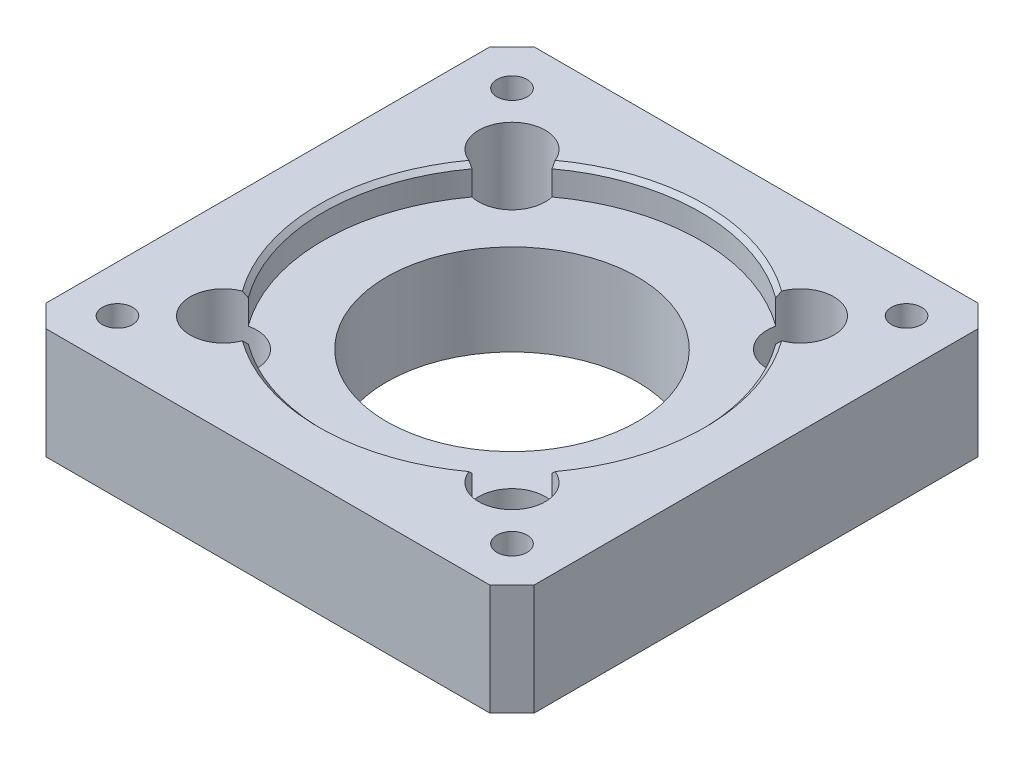
from build123d import *

# Parameters (mm, degrees)
SKETCH_1_W                     = 110
SKETCH_1_H                     = 110
EXTRUDE_1_DEPTH                = 25
SKETCH_3_R                     = 31.25
SKETCH_3_R_2                   = 28.25
EXTRUDE_2_DEPTH                = 2
SKETCH_4_R                     = 28.25
CUT_EXTRUDE_1_DEPTH            = 82.700673192
SKETCH_5_R                     = 42.5
CUT_EXTRUDE_2_DEPTH            = 6.5
HOLE_WIZARD_M8_1_D             = 6.8
HOLE_WIZARD_M8_1_DEPTH         = 19.75
HOLE_WIZARD_M8_1_TIP           = 2.042926105
HOLE_WIZARD_M8_1_2_D           = 9
HOLE_WIZARD_M8_1_2_CBORE_D     = 15
HOLE_WIZARD_M8_1_2_CBORE_DEPTH = 18
CHAMFER_1_SIZE                 = 5
CHAMFER_2_SIZE                 = 1
CHAMFER_3_SIZE                 = 0.5


with BuildPart() as part:
    # 草图1 → 凸台-拉伸1 (new body)
    with BuildSketch(Plane(origin=(0, 0, 0), x_dir=(1, 0, 0), z_dir=(0, 1, 0))):
        Rectangle(SKETCH_1_W, SKETCH_1_H)
    extrude(amount=EXTRUDE_1_DEPTH)

    # 草图3 → 凸台-拉伸2 (add)
    with BuildSketch(Plane.XZ):
        with Locations(Location((0, 0, 0), (0, 0, 270))):
            Circle(SKETCH_3_R)
        with Locations(Location((0, 0, 0), (0, 0, 270))):
            Circle(SKETCH_3_R_2, mode=Mode.SUBTRACT)
    extrude(amount=EXTRUDE_2_DEPTH)

    # 草图4 → 切除-拉伸1 (cut, through all)
    with BuildSketch(Plane.XZ):
        with Locations(Location((0, 0, 0), (0, 0, 270))):
            Circle(SKETCH_4_R)
    extrude(amount=-CUT_EXTRUDE_1_DEPTH, mode=Mode.SUBTRACT)

    # 草图5 → 切除-拉伸2 (cut)
    with BuildSketch(Plane(origin=(0, 25, 0), x_dir=(1, 0, 0), z_dir=(0, 1, 0))):
        with Locations(Location((0, 0, 0), (0, 0, 270))):
            Circle(SKETCH_5_R)
    extrude(amount=-CUT_EXTRUDE_2_DEPTH, mode=Mode.SUBTRACT)

    # Hole Wizard M8 _1
    with Locations(Plane(origin=(0, 25, 0), x_dir=(1, 0, 0), z_dir=(0, 1, 0))):
        with Locations((-44.45, 44.45), (0, 0), (44.45, 44.45), (-44.45, -44.45), (44.45, -44.45)):
            Hole(HOLE_WIZARD_M8_1_D / 2, depth=HOLE_WIZARD_M8_1_DEPTH)
            with Locations((0, 0, -(HOLE_WIZARD_M8_1_DEPTH + HOLE_WIZARD_M8_1_TIP / 2))):  # 118° drill point
                Cone(0, HOLE_WIZARD_M8_1_D / 2, HOLE_WIZARD_M8_1_TIP, mode=Mode.SUBTRACT)

    # Hole Wizard M8 _1 2 (through all)
    with Locations(Plane(origin=(0, 25, 0), x_dir=(1, 0, 0), z_dir=(0, 1, 0))):
        with Locations((-32.5, 32.5), (0, 0), (32.5, 32.5), (-32.5, -32.5), (32.5, -32.5)):
            CounterBoreHole(HOLE_WIZARD_M8_1_2_D / 2, HOLE_WIZARD_M8_1_2_CBORE_D / 2, HOLE_WIZARD_M8_1_2_CBORE_DEPTH)

    # 倒角1
    chamfer_1_edges = [part.edges().sort_by_distance(p)[0] for p in [
        (55, 12.5, 55),
        (-55, 12.5, 55),
        (-55, 12.5, -55),
        (55, 12.5, -55),
    ]]
    chamfer(chamfer_1_edges, length=CHAMFER_1_SIZE)

    # 倒角2
    chamfer_2_edges = [part.edges().sort_by_distance(p)[0] for p in [
        (-42.5, 25, 0),
        (42.5, 25, 0),
        (0, 25, 42.5),
        (0, 25, -42.5),
    ]]
    chamfer(chamfer_2_edges, length=CHAMFER_2_SIZE)

    # 倒角3
    chamfer_3_edges = [part.edges().sort_by_distance(p)[0] for p in [
        (0, -2, 31.25),
    ]]
    chamfer(chamfer_3_edges, length=CHAMFER_3_SIZE)


solid = part.part
